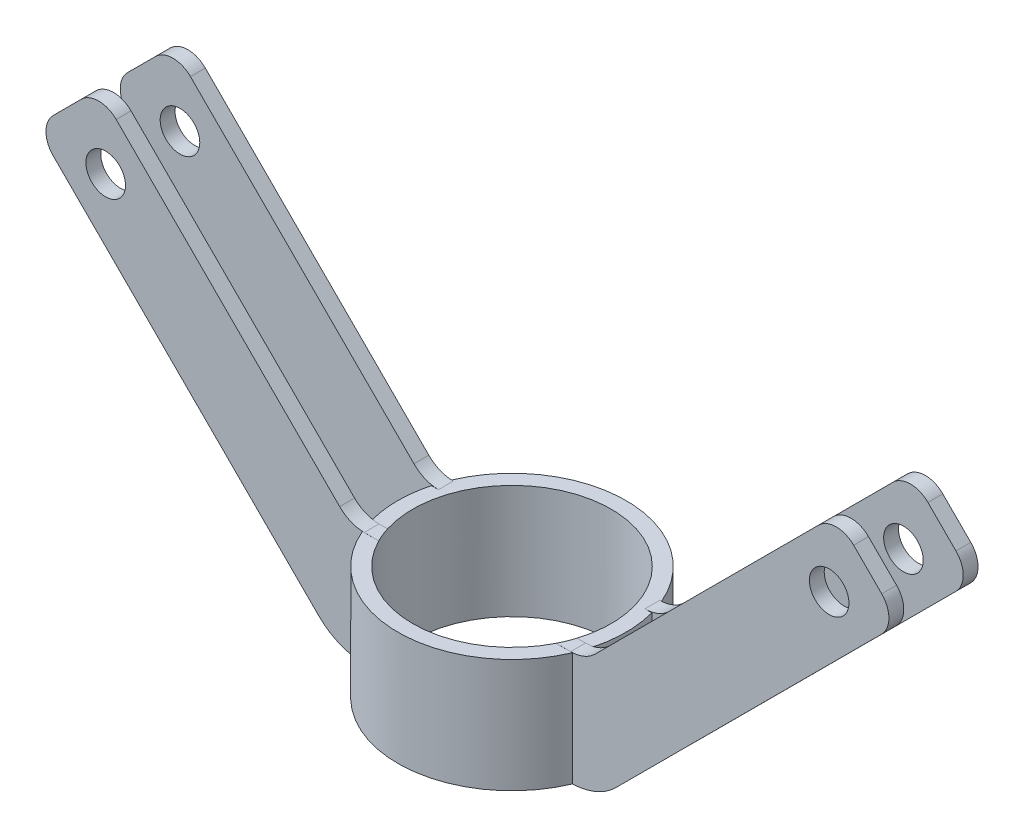
from build123d import *

# Parameters (mm, degrees)
SKETCH1_R               = 4
BOSS_EXTRU_1_DEPTH      = 3
SKETCH2_R               = 4
BOSS_EXTRU_2_DEPTH      = 3
CUT_EXTRUDE1_DEPTH      = 10
CUT_EXTRUDE1_DEPTH_BACK = 100.231025361
SKETCH3_R               = 20.05
BOSS_EXTRU_3_REACH      = 101.231
SKETCH5_R               = 23.05
SKETCH5_R_2             = 20.05


with BuildPart() as part:
    # Sketch1 → Boss.-Extru.1 (new body)
    with BuildSketch(Plane.XY):
        with BuildLine():
            Line((-83.689862838, 93.775756105), (-30.050252532, 40.136145798))
            ThreePointArc((-30.050252532, 40.136145798), (-25.832748997, 37.318100031), (-20.857864376, 36.328533954))
            Line((-20.857864376, 36.328533954), (20.857864376, 36.328533954))
            ThreePointArc((20.857864376, 36.328533954), (25.832748997, 37.318100031), (30.050252532, 40.136145798))
            Line((30.050252532, 40.136145798), (83.689862838, 93.775756105))
            ThreePointArc((83.689862838, 93.775756105), (85.154328933, 97.311290011), (83.689862838, 100.846823917))
            Line((83.689862838, 100.846823917), (78.033008589, 106.503678166))
            ThreePointArc((78.033008589, 106.503678166), (74.497474683, 107.96814426), (70.961940777, 106.503678166))
            Line((70.961940777, 106.503678166), (25.807611845, 61.349349234))
            ThreePointArc((25.807611845, 61.349349234), (23.536648403, 59.831939975), (20.857864376, 59.299096702))
            Line((20.857864376, 59.299096702), (-20.857864376, 59.299096702))
            ThreePointArc((-20.857864376, 59.299096702), (-23.536648403, 59.831939975), (-25.807611845, 61.349349234))
            Line((-25.807611845, 61.349349234), (-70.961940777, 106.503678166))
            ThreePointArc((-70.961940777, 106.503678166), (-74.497474683, 107.96814426), (-78.033008589, 106.503678166))
            Line((-78.033008589, 106.503678166), (-83.689862838, 100.846823917))
            ThreePointArc((-83.689862838, 100.846823917), (-85.154328933, 97.311290011), (-83.689862838, 93.775756105))
        make_face()
        with Locations((-73.083261121, 95.897076449)):
            Circle(SKETCH1_R, mode=Mode.SUBTRACT)
        with Locations(Location((73.083261121, 95.897076449, 0), (0, 0, 180))):
            Circle(SKETCH1_R, mode=Mode.SUBTRACT)
    extrude(amount=BOSS_EXTRU_1_DEPTH)


with BuildPart() as body_2:
    # Sketch2 → Boss.-Extru.2 (new body)
    with BuildSketch(Plane(origin=(0, 0, -12), x_dir=(-1, 0, 0), z_dir=(0, 0, -1))):
        with BuildLine():
            Line((-25.814562691, 61.342398387), (-70.968891623, 106.49672732))
            ThreePointArc((-70.968891623, 106.49672732), (-74.504425529, 107.961193414), (-78.039959435, 106.49672732))
            Line((-78.039959435, 106.49672732), (-83.696813685, 100.839873071))
            ThreePointArc((-83.696813685, 100.839873071), (-85.161279779, 97.304339165), (-83.696813685, 93.768805259))
            Line((-83.696813685, 93.768805259), (-30.057203378, 40.129194952))
            ThreePointArc((-30.057203378, 40.129194952), (-25.839699843, 37.311149185), (-20.864815223, 36.321583107))
            Line((-20.864815223, 36.321583107), (20.85091353, 36.321583107))
            ThreePointArc((20.85091353, 36.321583107), (25.825798151, 37.311149185), (30.043301685, 40.129194952))
            Line((30.043301685, 40.129194952), (83.682911992, 93.768805259))
            ThreePointArc((83.682911992, 93.768805259), (85.147378086, 97.304339165), (83.682911992, 100.839873071))
            Line((83.682911992, 100.839873071), (78.026057743, 106.49672732))
            ThreePointArc((78.026057743, 106.49672732), (74.490523837, 107.961193414), (70.954989931, 106.49672732))
            Line((70.954989931, 106.49672732), (25.800660998, 61.342398387))
            ThreePointArc((25.800660998, 61.342398387), (23.529697556, 59.824989128), (20.85091353, 59.292145856))
            Line((20.85091353, 59.292145856), (-20.864815223, 59.292145856))
            ThreePointArc((-20.864815223, 59.292145856), (-23.543599249, 59.824989128), (-25.814562691, 61.342398387))
        make_face()
        with Locations((-73.090211967, 95.890125602)):
            Circle(SKETCH2_R, mode=Mode.SUBTRACT)
        with Locations(Location((73.076310274, 95.890125602, 0), (0, 0, 180))):
            Circle(SKETCH2_R, mode=Mode.SUBTRACT)
    extrude(amount=BOSS_EXTRU_2_DEPTH)


with BuildPart() as cut_extrude1_tool:
    # Sketch3 → Cut-Extrude1 (new, two sides: drawn at the far end of the back side and taken through both)
    with BuildSketch(Plane(origin=(0, 59.292145856, 0), x_dir=(1, 0, 0), z_dir=(0, 1, 0)).offset(-CUT_EXTRUDE1_DEPTH_BACK)):
        with Locations((-0.00205312, 6.000001678)):
            Circle(SKETCH3_R)
    extrude(amount=CUT_EXTRUDE1_DEPTH + CUT_EXTRUDE1_DEPTH_BACK)


with BuildPart() as part_1:
    add(part.part)

    # Cut-Extrude1: cut by cut_extrude1_tool
    add(cut_extrude1_tool.part, mode=Mode.SUBTRACT)


with BuildPart() as body_2_1:
    add(body_2.part)

    # Cut-Extrude1: cut by cut_extrude1_tool
    add(cut_extrude1_tool.part, mode=Mode.SUBTRACT)


with BuildPart() as cut_extrude1_piece_1:
    # of the separate pieces the step leaves, piece 1, a body of its own (cut_extrude1_pieces)
    add(part_1.part.solids().sort_by_distance((19.129138162, 36.328533954, 0))[0])


with BuildPart() as cut_extrude1_piece_2:
    # of the separate pieces the step leaves, piece 2, a body of its own (cut_extrude1_pieces)
    add(part_1.part.solids().sort_by_distance((-83.689862838, 93.775756105, 0))[0])


with BuildPart() as cut_extrude1_piece_1_of_body_2:
    # of the separate pieces the step leaves, piece 1, a body of its own (cut_extrude1_pieces_of_body_2)
    add(body_2_1.part.solids().sort_by_distance((25.814562691, 61.342398387, -12))[0])


with BuildPart() as cut_extrude1_piece_2_of_body_2:
    # of the separate pieces the step leaves, piece 2, a body of its own (cut_extrude1_pieces_of_body_2)
    add(body_2_1.part.solids().sort_by_distance((-20.85091353, 59.292145856, -12))[0])

    # Boss.-Extru.3: up to this face of the body (flat: up to its plane)
    boss_extru_3_end = Plane(cut_extrude1_piece_2_of_body_2.part.faces().sort_by_distance((-19.684947548, 36.321583107, -13.633103381))[0])
    # Sketch5 → Boss.-Extru.3 (add, up to the picked face)
    with BuildSketch(Plane(origin=(0, 59.292145856, 0), x_dir=(1, 0, 0), z_dir=(0, 1, 0)), mode=Mode.PRIVATE) as boss_extru_3_sk1:
        with Locations(Location((-0.00205312, 6.000001678, 0), (0, 0, 180))):
            Circle(SKETCH5_R)
        with Locations(Location((-0.00205312, 6.000001678, 0), (0, 0, 342.587320704))):
            Circle(SKETCH5_R_2, mode=Mode.SUBTRACT)
    boss_extru_3_tool1 = split(extrude(boss_extru_3_sk1.sketch, amount=-BOSS_EXTRU_3_REACH, mode=Mode.PRIVATE), bisect_by=boss_extru_3_end, keep=Keep.BOTH, mode=Mode.PRIVATE)

    add(cut_extrude1_piece_1.part)  # Boss.-Extru.3 merges Cut-Extrude1 piece 1

    add(cut_extrude1_piece_2.part)  # Boss.-Extru.3 merges Cut-Extrude1 piece 2

    add(cut_extrude1_piece_1_of_body_2.part)  # Boss.-Extru.3 merges Cut-Extrude1 piece 1 of body 2
    add(boss_extru_3_tool1.solids().sort_by(Axis((22.395994, 59.292146, -6.000002), (0, -1, 0)))[0])


solid = cut_extrude1_piece_2_of_body_2.part
